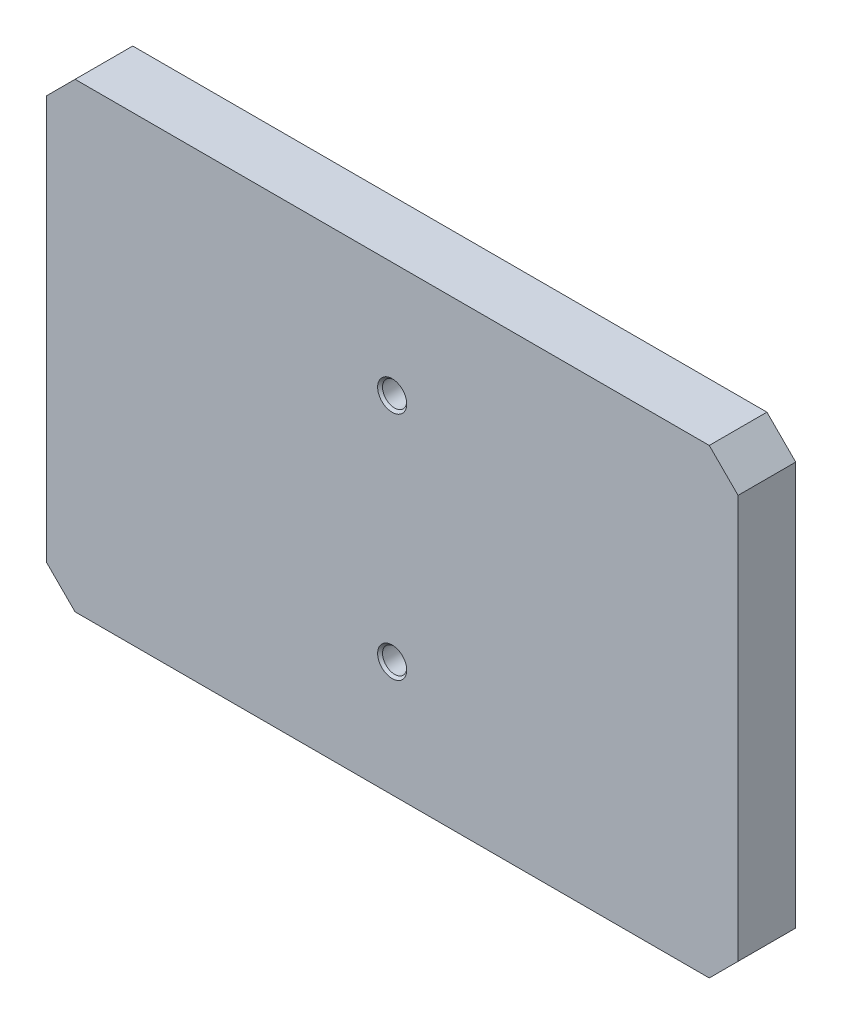
from build123d import *

# Parameters (mm, degrees)
SKETCH_1_W                   = 120
SKETCH_1_H                   = 80
EXTRUDE_1_DEPTH              = 10
CHAMFER_1_SIZE               = 5
HOLE_WIZARD_M5_1_D           = 4.2
HOLE_WIZARD_M5_1_DEPTH       = 14
HOLE_WIZARD_M5_1_CSINK_D     = 5.05
HOLE_WIZARD_M5_1_CSINK_ANGLE = 90
HOLE_WIZARD_M5_1_TIP         = 1.2618073


with BuildPart() as part:
    # 草图1 → 凸台-拉伸1 (new body)
    with BuildSketch(Plane.XY):
        Rectangle(SKETCH_1_W, SKETCH_1_H)
    extrude(amount=EXTRUDE_1_DEPTH)

    # 倒角1
    chamfer_1_edges = [part.edges().sort_by_distance(p)[0] for p in [
        (60, -40, 5),
        (-60, -40, 5),
        (-60, 40, 5),
        (60, 40, 5),
    ]]
    chamfer(chamfer_1_edges, length=CHAMFER_1_SIZE)

    # M5 螺纹孔1
    with Locations(Plane(origin=(0, 20, 10), x_dir=(1, 0, 0), z_dir=(0, 0, 1))):
        with Locations((0, 0), (0, -40)):
            CounterSinkHole(HOLE_WIZARD_M5_1_D / 2, HOLE_WIZARD_M5_1_CSINK_D / 2, depth=HOLE_WIZARD_M5_1_DEPTH, counter_sink_angle=HOLE_WIZARD_M5_1_CSINK_ANGLE)
            with Locations((0, 0, -(HOLE_WIZARD_M5_1_DEPTH + HOLE_WIZARD_M5_1_TIP / 2))):  # 118° drill point
                Cone(0, HOLE_WIZARD_M5_1_D / 2, HOLE_WIZARD_M5_1_TIP, mode=Mode.SUBTRACT)


solid = part.part
